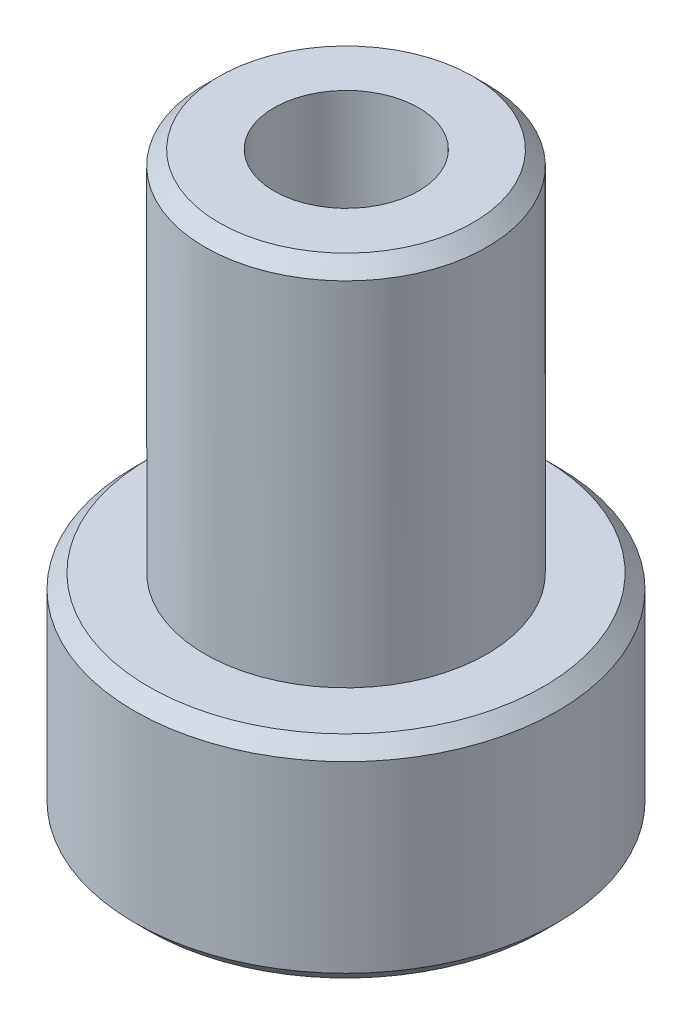
SolidWorks part; units mm, degrees
ref_plane "Front Plane" through (0, 0, 0) normal (0, 0, 1) x (1, 0, 0)
ref_plane "Top Plane" through (0, 0, 0) normal (0, 1, 0) x (1, 0, 0)
ref_plane "Right Plane" through (0, 0, 0) normal (1, 0, 0) x (0, 0, -1)
sketch "Sketch1" plane through (0, 0, 0) normal (0, 1, 0) x (1, 0, 0)
  circle A0 centre (0, 0) radius 2
  dimension "D1" = 4
extrude "Boss-Extrude1" add sketch "Sketch1" along normal blind 8.2
hole_wizard "M2.5 Tapped Hole1" positions "Sketch7" profile "Sketch6" tap size "M2.5" standard "Gb"
sketch "Sketch7" plane through (0, 8.2, 0) normal (0, 1, 0) x (1, 0, 0)
  point P0 (0, 0.0042)
sketch "Sketch6" plane through (0, 8.2, -0.0042) normal (1, 0, 0) x (0, 0, 1)
  line L0 (0, 0) -> (0, 6.9659)
  line L1 (0, 6.9659) -> (1.025, 6.35)
  line L2 (1.025, 6.35) -> (1.025, 0)
  line L5 (1.025, 0) -> (0, 0)
  line L10 (0, 6.9659) -> (-1.025, 6.35) construction
  line L11 (0, -6.35) -> (0, 107.95) construction
  dimension "螺纹孔钻头直径" = 2.05
  dimension "螺纹孔钻头深度" = 6.35
  dimension "导头角度" = 118
cosmetic thread "Cosmetic Thread1" parameters "D1"=5, "D2"=2.5
sketch "Sketch8" plane through (0, 0, 0) normal (0, -1, 0) x (1, 0, 0)
  circle A0 centre (0, 0) radius 3
  dimension "D1" = 6
extrude "Boss-Extrude2" add sketch "Sketch8" against normal blind 3
chamfer "Chamfer1" distance 0.2 angle 45 1 edges at (0, 8.2, 2)
chamfer "Chamfer2" distance 0.2 angle 45 2 edges at (0, 0, -3) (0, 3, -3)
